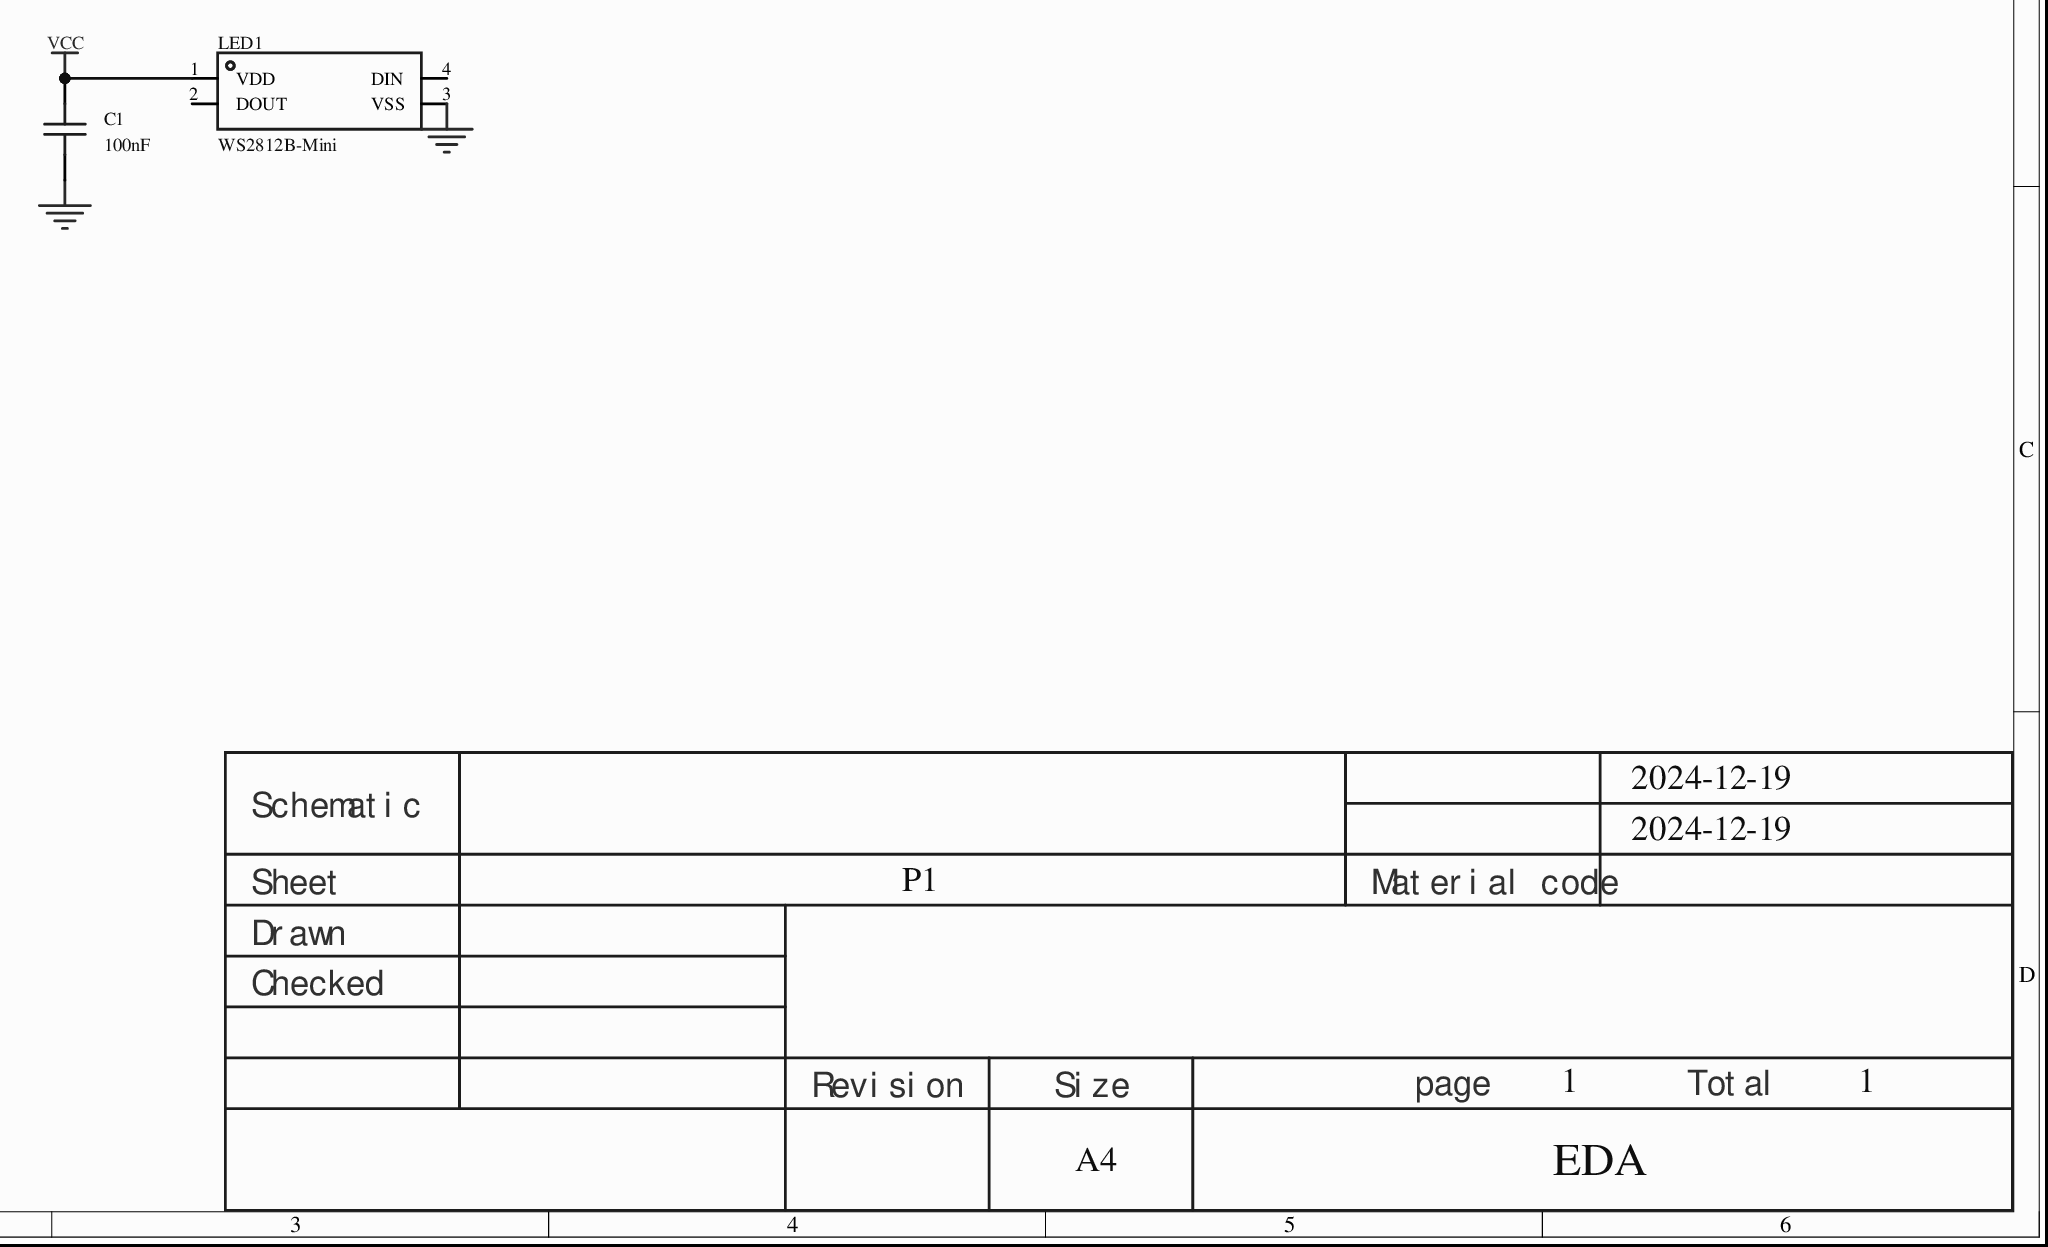
[diagram p0: MISC89036-3.schdoc]
# Altium project MISC89036-2.PrjPcb
1 sheet, 2 parts. Net scope: global (net labels, ports and power ports of the same name join across sheets).
Board file: MISC89036.pcbdoc

## Sheet MISC89036-3.schdoc
size 297 x 209 mm; Version: V1.0; @Project Name: MISC89036; @Page Count: 1; @Update Date: 2024-12-19; @Create Date: 2024-12-19; @Schematic Name: MISC89036; @Page No: 1; @Board Name: MISC89036; @Create Time: 16:49:47; @Update Time: 16:49:47

### Parts
C1  100nF  [C0603]
LED1  WS2812B-Mini  [LED-SMD_4P-L3.5-W3.5-TL_WS2812B]

### Nets
GND: C1.1 LED1.3(VSS)
VCC: C1.2 LED1.1(VDD)

Not connected (* = marked no-connect by the designer): LED1 2(DOUT) 4(DIN)

### Notes on the sheet
- 2024-12-19
- Schematic
- Sheet
- P1
- Material code
- Checked
- Drawn
- Revision
- Size
- A4
- page
- 1
- EDA
- Total

### Library data of the parts
C1 = CAP_0603: ConvertToPcb: yes; SymbolName: CapAcitance; ModelId: ac125912035d415993ca9572d50418b1; ModelName: C0603_L1.6-W0.8-H0.8; ModelTransform: 62.992,31.496,0,0,0,0,0,0,0; Device: CAP_0603; AddInBom: yes; Supplier Footprint: 0603; FootprintName: C0603; Value: 100nF
LED1 = WS2812B-Mini: (moisture sensitive: see datasheet for details); Manufacturer: worldsemi; Symbol: WS2812B-3535; AddInBom: yes; ModelId: 9feeb2fcd1804ea1b8a106e0513d23f0; ModelName: LED3535-4P_L3.5-W3.5-H1.9-LS3.7; ModelTransform: 145.669,145.669,0,180,0,0,0,0,0; Device: WS2812B-Mini; LCSC Part Name: WS2812B-Mini; SupplierPart: C114583; ManufacturerPart: WS2812B-Mini; Supplier Footprint: SMD3535; JLCPCB Part Class: JLCPCB Part Class  Extended Library; Datasheet: https://atta.szlcsc.com/upload/public/pdf/source/20190620/C114583_ECCAEB884D1CBA01F5696FFC90F90D84.pdf; Supplier: LCSC; ConvertToPcb: yes; FootprintName: LED-SMD_4P-L3.5-W3.5-TL_WS2812B